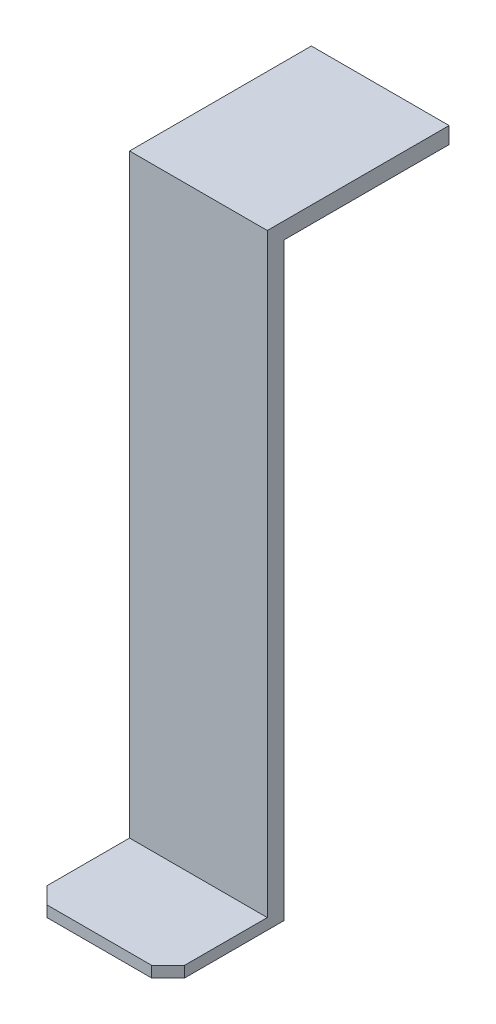
from build123d import *

# Parameters (mm, degrees)
SKETCH_1_W      = 25
SKETCH_1_H      = 110
EXTRUDE_1_DEPTH = 3
SKETCH_3_W      = 25
SKETCH_3_H      = 2
EXTRUDE_2_DEPTH = 18
SKETCH_4_W      = 25
SKETCH_4_H      = 3
EXTRUDE_3_DEPTH = 30
CHAMFER_1_SIZE  = 3


with BuildPart() as part:
    # 草图1 → 凸台-拉伸1 (new body)
    with BuildSketch(Plane.XY):
        Rectangle(SKETCH_1_W, SKETCH_1_H)
    extrude(amount=EXTRUDE_1_DEPTH)

    # 草图3 → 凸台-拉伸2 (add)
    with BuildSketch(Plane.XY.offset(3)):
        with Locations((0, -54)):
            Rectangle(SKETCH_3_W, SKETCH_3_H)
    extrude(amount=EXTRUDE_2_DEPTH)

    # 草图4 → 凸台-拉伸3 (add)
    with BuildSketch(Plane(origin=(0, 0, 0), x_dir=(-1, 0, 0), z_dir=(0, 0, -1))):
        with Locations((0, 53.5)):
            Rectangle(SKETCH_4_W, SKETCH_4_H)
    extrude(amount=EXTRUDE_3_DEPTH)

    # 倒角1
    chamfer_1_edges = [part.edges().sort_by_distance(p)[0] for p in [
        (-12.5, -54, 21),
        (12.5, -54, 21),
    ]]
    chamfer(chamfer_1_edges, length=CHAMFER_1_SIZE)


solid = part.part
